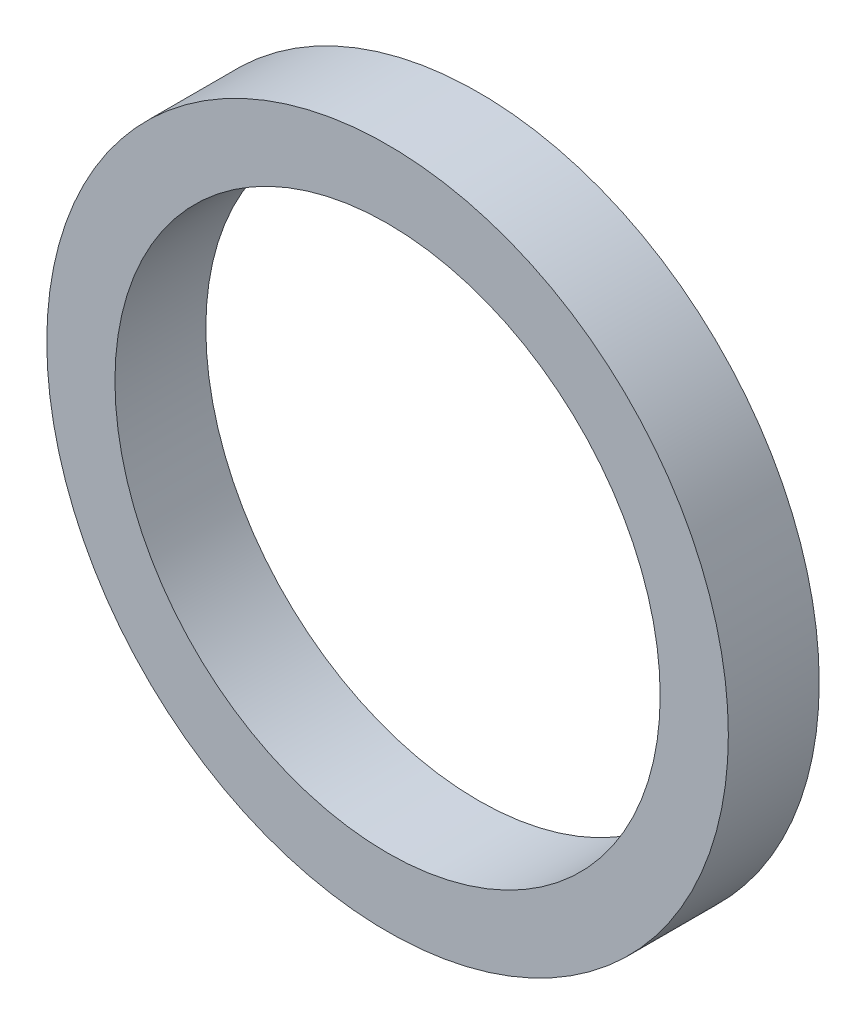
SolidWorks part; units mm, degrees
ref_plane "Front Plane" through (0, 0, 0) normal (0, 0, 1) x (1, 0, 0)
ref_plane "Top Plane" through (0, 0, 0) normal (0, 1, 0) x (1, 0, 0)
ref_plane "Right Plane" through (0, 0, 0) normal (1, 0, 0) x (0, 0, -1)
sketch "Sketch2" plane through (0, 0, 0) normal (0, 0, 1) x (1, 0, 0)
  circle A0 centre (0, 0) radius 7.5
  circle A1 centre (0, 0) radius 6
  dimension "D1" = 12
  dimension "D2" = 15
extrude "Boss-Extrude1" add sketch "Sketch2" along normal blind 2
